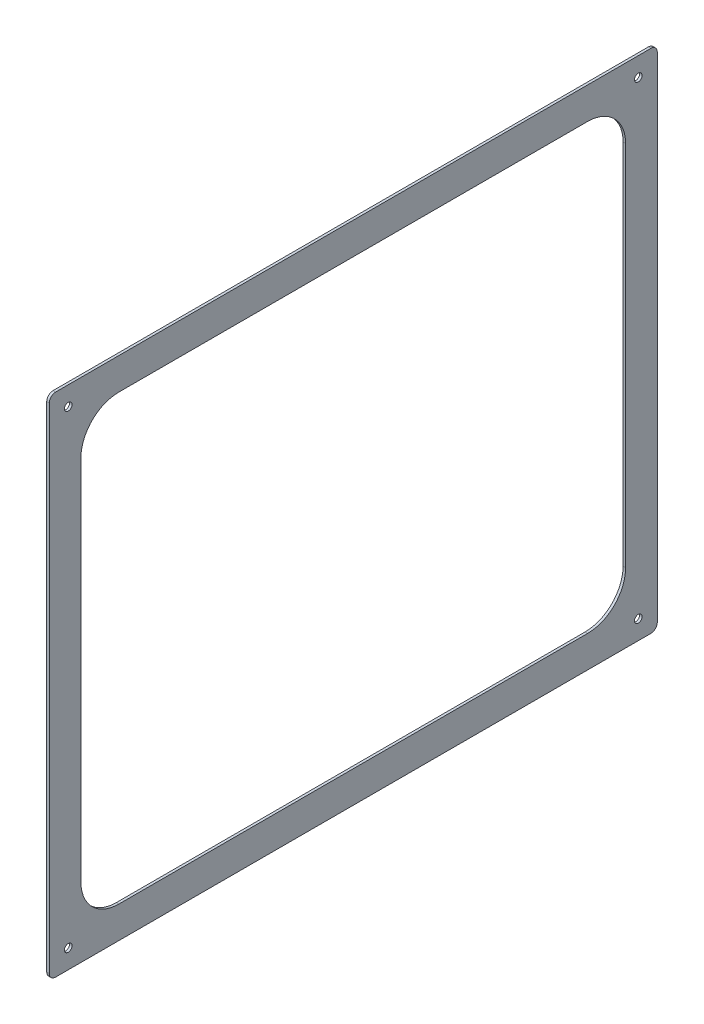
SolidWorks part; units mm, degrees
ref_plane "前视基准面" through (0, 0, 0) normal (0, 0, 1) x (1, 0, 0)
ref_plane "上视基准面" through (0, 0, 0) normal (0, 1, 0) x (1, 0, 0)
ref_plane "右视基准面" through (0, 0, 0) normal (1, 0, 0) x (0, 0, -1)
sketch "草图1" plane through (0, 0, 0) normal (1, 0, 0) x (0, 0, -1)
  line L0 (0, 200) -> (0, 0) construction
  line L1 (-240, 200) -> (240, 200)
  line L2 (-240, 200) -> (-240, -200)
  line L3 (-240, -200) -> (240, -200)
  line L4 (240, 200) -> (240, -200)
  line L5 (0, 0) -> (240, 0) construction
  dimension "D1" = 480
  dimension "D2" = 400
extrude "凸台-拉伸1" add sketch "草图1" along normal blind 2
sketch "草图2" plane through (2, 0, 0) normal (1, 0, 0) x (0, 0, -1)
  line L0 (0, 131.9543) -> (0, 0) construction
  line L1 (0, 0) -> (347.0268, 0) construction
  circle A0 centre (-225, 185) radius 3
  circle A1 centre (225, 185) radius 3
  circle A2 centre (-225, -185) radius 3
  circle A3 centre (225, -185) radius 3
  dimension "D1" = 6
  dimension "D2" = 450
  dimension "D3" = 370
extrude "切除-拉伸1" cut sketch "草图2" against normal through all
fillet "圆角1" radius 5 4 edges at (1, -200, 240) (1, -200, -240) (1, 200, -240) (1, 200, 240)
sketch "草图3" plane through (2, 0, 0) normal (1, 0, 0) x (0, 0, -1)
  line L0 (0, 234.3194) -> (0, 0) construction
  line L1 (-215, 175) -> (215, 175)
  line L2 (-215, 175) -> (-215, -175)
  line L3 (-215, -175) -> (215, -175)
  line L4 (215, 175) -> (215, -175)
  line L5 (0, 0) -> (371.0835, 0) construction
  dimension "D1" = 350
  dimension "D2" = 430
extrude "切除-拉伸2" cut sketch "草图3" against normal through all
fillet "圆角2" radius 30 4 edges at (1, -175, 215) (1, -175, -215) (1, 175, -215) (1, 175, 215)
